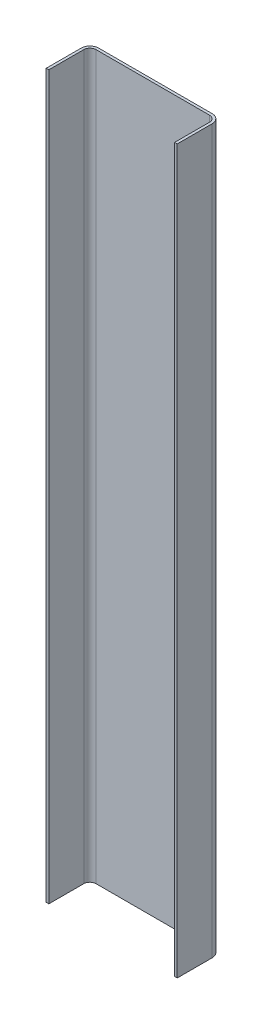
SolidWorks part; units mm, degrees
ref_plane "Front Plane" through (0, 0, 0) normal (0, 0, 1) x (1, 0, 0)
ref_plane "Top Plane" through (0, 0, 0) normal (0, 1, 0) x (1, 0, 0)
ref_plane "Right Plane" through (0, 0, 0) normal (1, 0, 0) x (0, 0, -1)
other "Configuration Table"
sketch "Sketch1" plane through (0, 0, 0) normal (0, 1, 0) x (1, 0, 0)
  line L1 (-65, 25) -> (65, 25)
  line L2 (-75, 15) -> (-75, -25)
  line L4 (75, 15) -> (75, -25)
  line L5 (-75, 25) -> (75, -25) construction
  line L6 (-75, -25) -> (75, 25) construction
  arc A0 (65, 25) -> (75, 15) centre (65, 15) cw
  arc A3 (-65, 25) -> (-75, 15) centre (-65, 15) ccw
  point P0 (0, 0)
  dimension "D3" = 10
  dimension "D1" = 150
  dimension "D2" = 50
extrude "Extrude-Thin1" add sketch "Sketch1" along normal mid plane 827 thin
